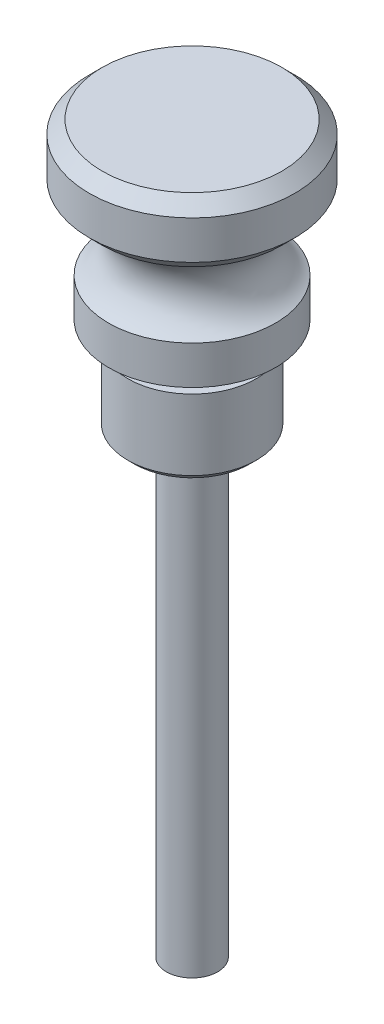
SolidWorks part; units mm, degrees
ref_plane "Front" through (0, 0, 0) normal (0, 0, 1) x (1, 0, 0)
ref_plane "Top" through (0, 0, 0) normal (0, 1, 0) x (1, 0, 0)
ref_plane "Right" through (0, 0, 0) normal (1, 0, 0) x (0, 0, -1)
sketch "Sketch1" plane through (0, 0, 0) normal (0, 0, 1) x (1, 0, 0)
  line L0 (4, -40) -> (4, -111)
  line L1 (16, 0) -> (16, -6)
  line L2 (0, 2) -> (14, 2)
  line L3 (14, 2) -> (16, 0)
  line L5 (0, -112) -> (2, -112)
  line L6 (0, 2) -> (0, -112)
  line L7 (14, -8) -> (16, -6)
  line L8 (13, -19) -> (13, -25)
  line L9 (13, -25) -> (6.5, -25)
  line L10 (6.5, -25) -> (6.5, -28)
  line L11 (6.5, -28) -> (10, -28)
  line L12 (10, -28) -> (10, -39)
  line L13 (2, -112) -> (4, -111)
  line L14 (4, -40) -> (9, -40)
  line L15 (9, -40) -> (10, -39)
  arc A0 (14, -8) -> (13, -19) centre (15.8356, -13.7123) ccw
  dimension "D7" = 6
  dimension "D2" = 6
  dimension "D3" = 14
  dimension "D4" = 71
  dimension "D8" = 2
  dimension "D9" = 6
  dimension "D11" = 3
  dimension "D13" = 11
revolve "Revolve1" add sketch "Sketch1" angle 360 about L6
scale "Scale 1" bodies to scale 101 scale about centroid uniform scaling yes scale factor 1.875
